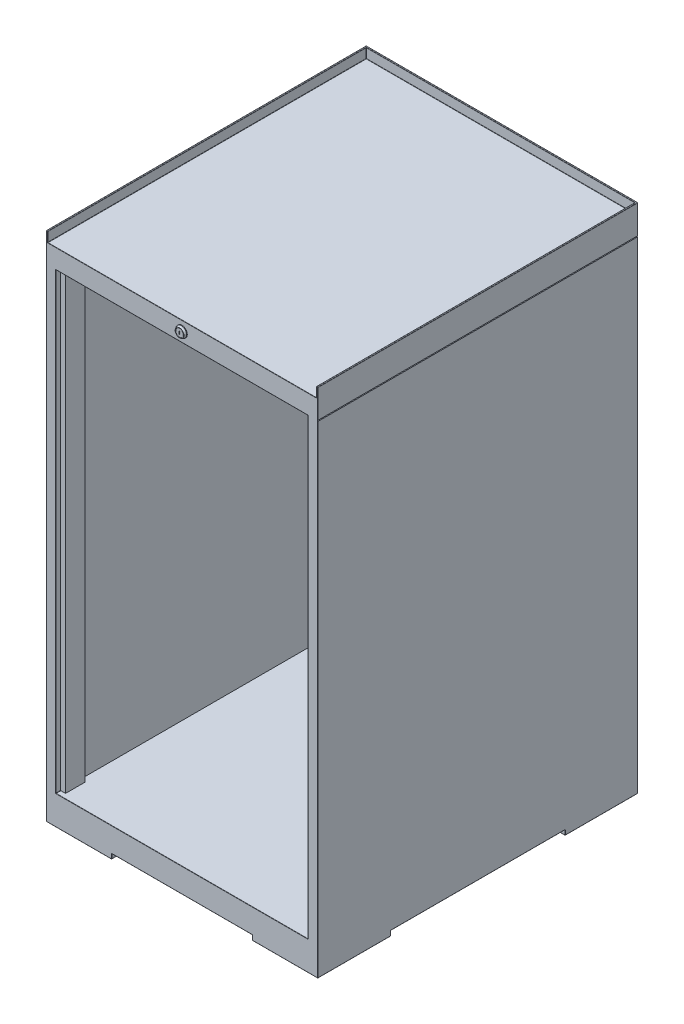
from build123d import *

# Parameters (mm, degrees)
SKETCH1_W             = 560
SKETCH1_H             = 1055
BOSS_EXTRUDE1_DEPTH   = 660
SKETCH2_W             = 554
SKETCH2_H             = 40
CUT_EXTRUDE1_DEPTH    = 657
SKETCH3_W             = 520
SKETCH3_H             = 935
CUT_EXTRUDE2_DEPTH    = 657
CUT_EXTRUDE3_DEPTH    = 10
FILETE1_R             = 1
SKETCH5_W             = 10
SKETCH5_H             = 40
BOSS_EXTRUDE2_DEPTH   = 935
CUT_EXTRUDE4_DEPTH    = 891.08777657
CUT_EXTRUDE5_DEPTH    = 1014.635166122
SKETCH9_R             = 11
BOSS_EXTRUDE3_DEPTH   = 1.5
SKETCH10_R            = 11
BOSS_EXTRUDE4_DEPTH   = 3.5
BOSS_EXTRUDE4_TAPER   = 30
SKETCH11_R            = 8
SKETCH11_R_2          = 7.75
CUT_EXTRUDE6_DEPTH    = 5
SKETCH12_W            = 2
SKETCH12_H            = 6
CUT_EXTRUDE7_DEPTH    = 0.5
FILETE2_R             = 0.5
TAPPED_HOLE_M61_D     = 5
TAPPED_HOLE_M61_DEPTH = 17
TAPPED_HOLE_M61_TIP   = 1.502151548


with BuildPart() as part:
    # Sketch1 → Boss-Extrude1 (new body)
    with BuildSketch(Plane.XY):
        Rectangle(SKETCH1_W, SKETCH1_H)
    extrude(amount=BOSS_EXTRUDE1_DEPTH)

    # Sketch2 → Cut-Extrude1 (cut)
    with BuildSketch(Plane.XY.offset(660)):
        with Locations((0, 527.5)):
            Rectangle(SKETCH2_W, SKETCH2_H)
    extrude(amount=-CUT_EXTRUDE1_DEPTH, mode=Mode.SUBTRACT)

    # Sketch3 → Cut-Extrude2 (cut)
    with BuildSketch(Plane.XY.offset(660)):
        Rectangle(SKETCH3_W, SKETCH3_H)
    extrude(amount=-CUT_EXTRUDE2_DEPTH, mode=Mode.SUBTRACT)

    # Sketch4 → Cut-Extrude3 (cut)
    with BuildSketch(Plane.XZ.offset(527.5)):
        Polygon((-145, 660), (-145, 510), (-280, 510), (-280, 150), (-145, 150), (-145, 0), (145, 0), (145, 150), (280, 150), (280, 510), (145, 510), (145, 660), align=None)
    extrude(amount=-CUT_EXTRUDE3_DEPTH, mode=Mode.SUBTRACT)

    # Filete1
    filete1_edges = [part.edges().sort_by_distance(p)[0] for p in [
        (-278.5, 527.5, 660),
        (278.5, 527.5, 660),
    ]]
    fillet(filete1_edges, radius=FILETE1_R)

    # Sketch5 → Boss-Extrude2 (add)
    with BuildSketch(Plane(origin=(0, -467.5, 0), x_dir=(1, 0, 0), z_dir=(0, 1, 0))):
        with Locations((-255, -630)):
            Rectangle(SKETCH5_W, SKETCH5_H)
        with Locations((255, -630)):
            Rectangle(SKETCH5_W, SKETCH5_H)
        with Locations((-255, -33)):
            Rectangle(SKETCH5_W, SKETCH5_H)
        with Locations((255, -33)):
            Rectangle(SKETCH5_W, SKETCH5_H)
    extrude(amount=BOSS_EXTRUDE2_DEPTH)

    # Sketch6 → Cut-Extrude4 (cut, through all)
    with BuildSketch(Plane.XY.offset(660)):
        Polygon((279, 467.5), (280, 468.5), (280, 466.5), align=None)
        Polygon((-279, 467.5), (-280, 468.5), (-280, 466.5), align=None)
    extrude(amount=-CUT_EXTRUDE4_DEPTH, mode=Mode.SUBTRACT)

    # Sketch7 → Cut-Extrude5 (cut, through all)
    with BuildSketch(Plane.ZY.offset(280)):
        Polygon((0, 468.5), (1, 467.5), (0, 466.5), align=None)
    extrude(amount=-CUT_EXTRUDE5_DEPTH, mode=Mode.SUBTRACT)

    # Sketch9 → Boss-Extrude3 (add)
    with BuildSketch(Plane.XY.offset(660)):
        with Locations((0, 487.5)):
            Circle(SKETCH9_R)
    extrude(amount=BOSS_EXTRUDE3_DEPTH)

    # Sketch10 → Boss-Extrude4 (add)
    with BuildSketch(Plane.XY.offset(661.5)):
        with Locations((0, 487.5)):
            Circle(SKETCH10_R)
    extrude(amount=BOSS_EXTRUDE4_DEPTH, taper=BOSS_EXTRUDE4_TAPER)

    # Sketch11 → Cut-Extrude6 (cut)
    with BuildSketch(Plane.XY.offset(665)):
        with Locations((0, 487.5)):
            Circle(SKETCH11_R)
        with Locations((0, 487.5)):
            Circle(SKETCH11_R_2, mode=Mode.SUBTRACT)
    extrude(amount=-CUT_EXTRUDE6_DEPTH, mode=Mode.SUBTRACT)

    # Sketch12 → Cut-Extrude7 (cut)
    with BuildSketch(Plane.XY.offset(665)):
        with Locations((0, 487.5)):
            Rectangle(SKETCH12_W, SKETCH12_H)
    extrude(amount=-CUT_EXTRUDE7_DEPTH, mode=Mode.SUBTRACT)

    # Filete2
    filete2_edges = [part.edges().sort_by_distance(p)[0] for p in [
        (-260, -467.5, 655),
        (260, 467.5, 655),
        (260, -467.5, 655),
        (-212.5, -527.5, 660),
        (280, 498, 0),
        (0, 527.5, 3),
        (280, 497.5, 660),
        (277, 517, 660),
        (-280, -30.5, 0),
        (-280, -30.5, 660),
        (0, 507.5, 660),
        (277, 517.5, 3),
        (277, 527.5, 331),
        (-277, 517.5, 3),
        (-277, 507.5, 331.5),
        (0, 507.5, 3),
        (277, 507.5, 331.5),
        (260, 0, 660),
        (0, 467.5, 660),
        (-260, 0, 660),
        (0, -467.5, 660),
        (280, -30.5, 660),
        (-212.5, -527.5, 0),
        (212.5, -527.5, 0),
        (212.5, -527.5, 660),
        (-280, 498, 0),
        (280, -527.5, 75),
        (-280, -527.5, 75),
        (0, 527.5, 0),
        (280, -30.5, 0),
        (0, -517.5, 660),
        (-145, -522.5, 660),
        (145, -517.5, 585),
        (145, -522.5, 660),
        (212.5, -517.5, 510),
        (145, -522.5, 510),
        (280, -517.5, 330),
        (280, -522.5, 510),
        (212.5, -517.5, 150),
        (280, -522.5, 150),
        (145, -517.5, 75),
        (145, -522.5, 150),
        (0, -517.5, 0),
        (145, -522.5, 0),
        (-145, -517.5, 75),
        (-145, -522.5, 0),
        (-212.5, -517.5, 150),
        (-145, -522.5, 150),
        (-280, -517.5, 330),
        (-280, -522.5, 150),
        (-212.5, -517.5, 510),
        (-280, -522.5, 510),
        (-145, -517.5, 585),
        (-145, -522.5, 510),
        (-145, -527.5, 585),
        (-212.5, -527.5, 510),
        (-212.5, -527.5, 150),
        (-145, -527.5, 75),
        (145, -527.5, 75),
        (212.5, -527.5, 150),
        (212.5, -527.5, 510),
        (145, -527.5, 585),
        (280, -527.5, 585),
        (-280, -527.5, 585),
        (-277, 517, 660),
        (-280, 497.5, 660),
        (277, 527.207106781, 659.707106781),
        (280, 527.5, 329.5),
        (-280, 527.5, 329.5),
        (-277, 527.5, 331),
        (280, 527.207106781, 659.707106781),
        (-280, 527.207106781, 659.707106781),
        (-277, 527.207106781, 659.707106781),
        (-260, 467.5, 655),
    ]]
    fillet(filete2_edges, radius=FILETE2_R)

    # Tapped Hole M61
    with Locations(Plane(origin=(0, 0, 0), x_dir=(-1, 0, 0), z_dir=(0, 0, -1))):
        with Locations((-197.25, 415), (-82.75, 415), (197.25, 415), (82.75, 415)):
            Hole(TAPPED_HOLE_M61_D / 2, depth=TAPPED_HOLE_M61_DEPTH)
            with Locations((0, 0, -(TAPPED_HOLE_M61_DEPTH + TAPPED_HOLE_M61_TIP / 2))):  # 118° drill point
                Cone(0, TAPPED_HOLE_M61_D / 2, TAPPED_HOLE_M61_TIP, mode=Mode.SUBTRACT)


solid = part.part
